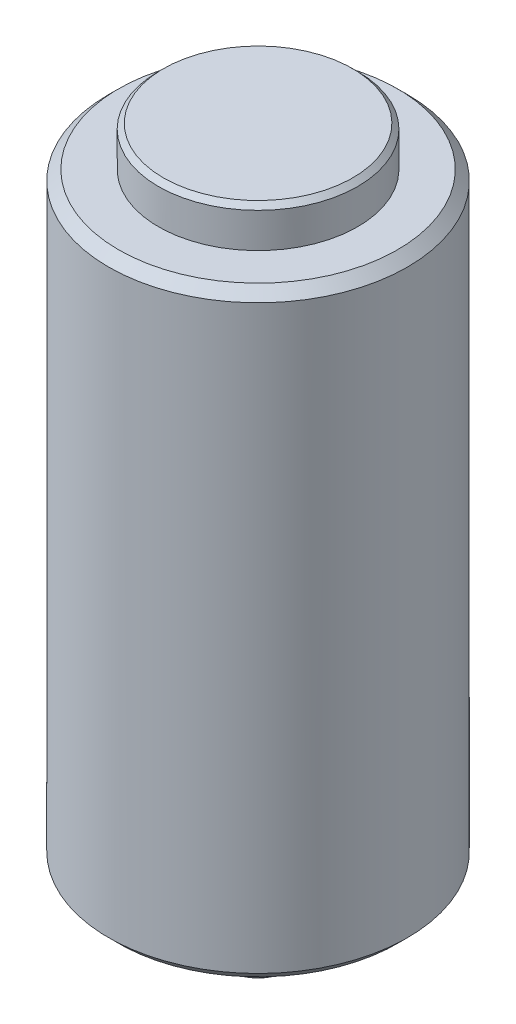
from build123d import *

# Parameters (mm, degrees)
CHAMFER1_SIZE = 1
CHAMFER2_SIZE = 0.5


with BuildPart() as part:
    # Sketch1 → Revolve1 (revolve)
    with BuildSketch(Plane.XY, mode=Mode.PRIVATE) as revolve1_sk:
        Polygon((486.666563646, -1172.870531067), (486.666563646, -1112.570531067), (481.666563646, -1112.570531067), (481.666563646, -1108.570531067), (471.666563646, -1108.570531067), (471.666563646, -1180.570531067), (475.916563646, -1180.570531067), (475.916563646, -1174.870531067), (477.916563646, -1174.870531067), (477.916563646, -1172.870531067), align=None)
    revolve(revolve1_sk.sketch.rotate(Axis((471.666563646, -1180.570531067, 0), (0, 1, 0)), 90), axis=Axis((471.666563646, -1180.570531067, 0), (0, 1, 0)))

    # Chamfer1
    chamfer1_edges = [part.edges().sort_by_distance(p)[0] for p in [
        (471.666563646, -1112.570531067, 15),
        (471.666563646, -1172.870531067, 15),
        (471.666563646, -1180.570531067, 4.25),
    ]]
    chamfer(chamfer1_edges, length=CHAMFER1_SIZE)

    # Chamfer2
    chamfer2_edges = [part.edges().sort_by_distance(p)[0] for p in [
        (471.666563646, -1108.570531067, 10),
        (471.666563646, -1174.870531067, 6.25),
    ]]
    chamfer(chamfer2_edges, length=CHAMFER2_SIZE)


solid = part.part
